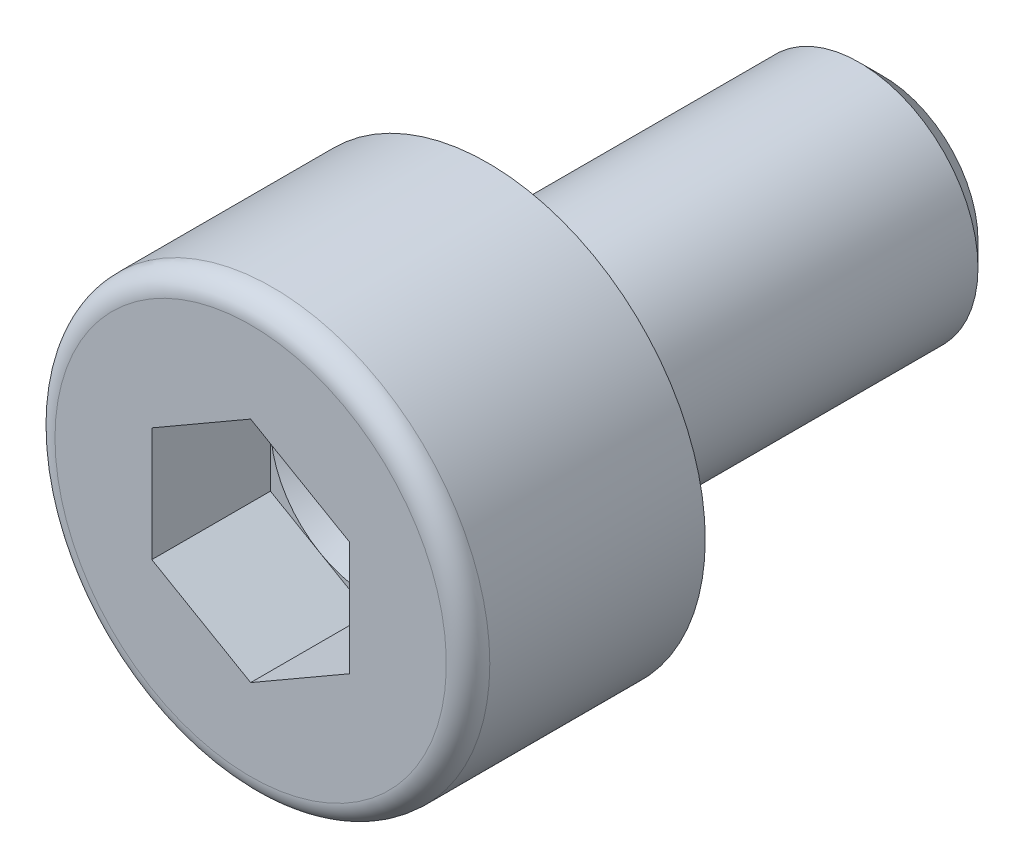
SolidWorks part; units mm, degrees
ref_plane "Front Plane" through (0, 0, 0) normal (0, 0, 1) x (1, 0, 0)
ref_plane "Top Plane" through (0, 0, 0) normal (0, 1, 0) x (1, 0, 0)
ref_plane "Right Plane" through (0, 0, 0) normal (1, 0, 0) x (0, 0, -1)
sketch "Sketch1" plane through (0, 0, 0) normal (1, 0, 0) x (0, 0, -1)
  line L0 (-3, 0) -> (5, 0) construction
  line L1 (-3, 0) -> (-3, 2.75)
  line L2 (-3, 2.75) -> (0, 2.75)
  line L3 (0, 2.75) -> (0, 1.5)
  line L4 (0, 1.5) -> (5, 1.5)
  line L5 (5, 1.5) -> (5, 0)
  point P3 (0, 1.5)
  point P8 (-1.5, 0)
  point P9 (0.125, 1.5)
  point P10 (5, 0.6)
  dimension "A" = 5.5
  dimension "E" = 3
  dimension "L" = 5
  dimension "M" = 3
  dimension "t" = 1.5
  dimension "r" = 0.125
  dimension "(d)" = 1.2
sketch "Sketch2" plane through (0, 0, 0) normal (0, 0, 1) x (1, 0, 0)
  line L1 (0, 1.4434) -> (-1.25, 0.7217)
  line L2 (-1.25, 0.7217) -> (-1.25, -0.7217)
  line L3 (-1.25, -0.7217) -> (0, -1.4434)
  line L4 (0, -1.4434) -> (1.25, -0.7217)
  line L5 (1.25, -0.7217) -> (1.25, 0.7217)
  line L6 (1.25, 0.7217) -> (0, 1.4434)
  circle A0 centre (0, 0) radius 1.25 construction
  dimension "B" = 2.5
sketch "Sketch3" plane through (0, 0, 0) normal (1, 0, 0) x (0, 0, -1)
  line L0 (-3, 0) -> (-3, 2.75) construction
  line L1 (-3, 2.75) -> (0, 2.75) construction
  line L2 (0, 1.5) -> (5, 1.5) construction
  line L3 (0, 2.75) -> (0, 1.5) construction
  line L5 (5, 1.5) -> (5, 0) construction
  line L6 (-3, 0.6) -> (-3, 2.75)
  line L7 (-3, 2.75) -> (0, 2.75)
  line L8 (0, 1.5) -> (5, 1.5)
  line L9 (0, 2.75) -> (0, 1.5)
  line L10 (5, 0.6) -> (-3, 0.6)
  line L11 (5, 1.5) -> (5, 0.6)
revolve "Revolve1" add sketch "Sketch3" angle 360 about L0
cosmetic thread "Cosmetic-Thread1" parameters "D1"=9.875, "D2"=2.55
sketch "Sketch4" plane through (0, 0, 3) normal (0, 0, 1) x (1, 0, 0)
  line L0 (0, 1.4434) -> (-1.25, 0.7217) construction
  line L1 (-1.25, 0.7217) -> (-1.25, -0.7217) construction
  line L2 (-1.25, -0.7217) -> (0, -1.4434) construction
  line L3 (0, -1.4434) -> (1.25, -0.7217) construction
  line L4 (1.25, -0.7217) -> (1.25, 0.7217) construction
  line L5 (1.25, 0.7217) -> (0, 1.4434) construction
  line L6 (0, 1.4434) -> (-1.25, 0.7217)
  line L7 (-1.25, 0.7217) -> (-1.25, -0.7217)
  line L8 (-1.25, -0.7217) -> (0, -1.4434)
  line L9 (0, -1.4434) -> (1.25, -0.7217)
  line L10 (1.25, -0.7217) -> (1.25, 0.7217)
  line L11 (1.25, 0.7217) -> (0, 1.4434)
extrude "Cut-Extrude1" cut sketch "Sketch4" against normal blind 1.5
fillet "Fillet1" radius 0.275 1 edges at (2.75, 0, 3)
chamfer "Chamfer1" distance 0.3 angle 45 1 edges at (1.5, 0, -5)
sketch "Sketch5" plane through (0, 0, 1.5) normal (0, 0, 1) x (1, 0, 0)
  line L6 (1.25, 0.7217) -> (0, 1.4434)
  line L7 (0, 1.4434) -> (-1.25, 0.7217)
  line L8 (-1.25, 0.7217) -> (-1.25, -0.7217)
  line L9 (-1.25, -0.7217) -> (0, -1.4434)
  line L10 (0, -1.4434) -> (1.25, -0.7217)
  line L11 (1.25, -0.7217) -> (1.25, 0.7217)
  line L12 (1.25, 0.7217) -> (0, 1.4434) construction
  line L13 (0, 1.4434) -> (-1.25, 0.7217) construction
  line L14 (-1.25, 0.7217) -> (-1.25, -0.7217) construction
  line L15 (-1.25, -0.7217) -> (0, -1.4434) construction
  line L16 (0, -1.4434) -> (1.25, -0.7217) construction
  line L17 (1.25, -0.7217) -> (1.25, 0.7217) construction
  circle A0 centre (0, 0) radius 1.25
  dimension "D1" = 0
extrude "Cut-Extrude2" cut sketch "Sketch5" against normal blind 10 draft 60
fillet "Fillet2" radius 0.125 1 edges at (1.5, 0, 0)
